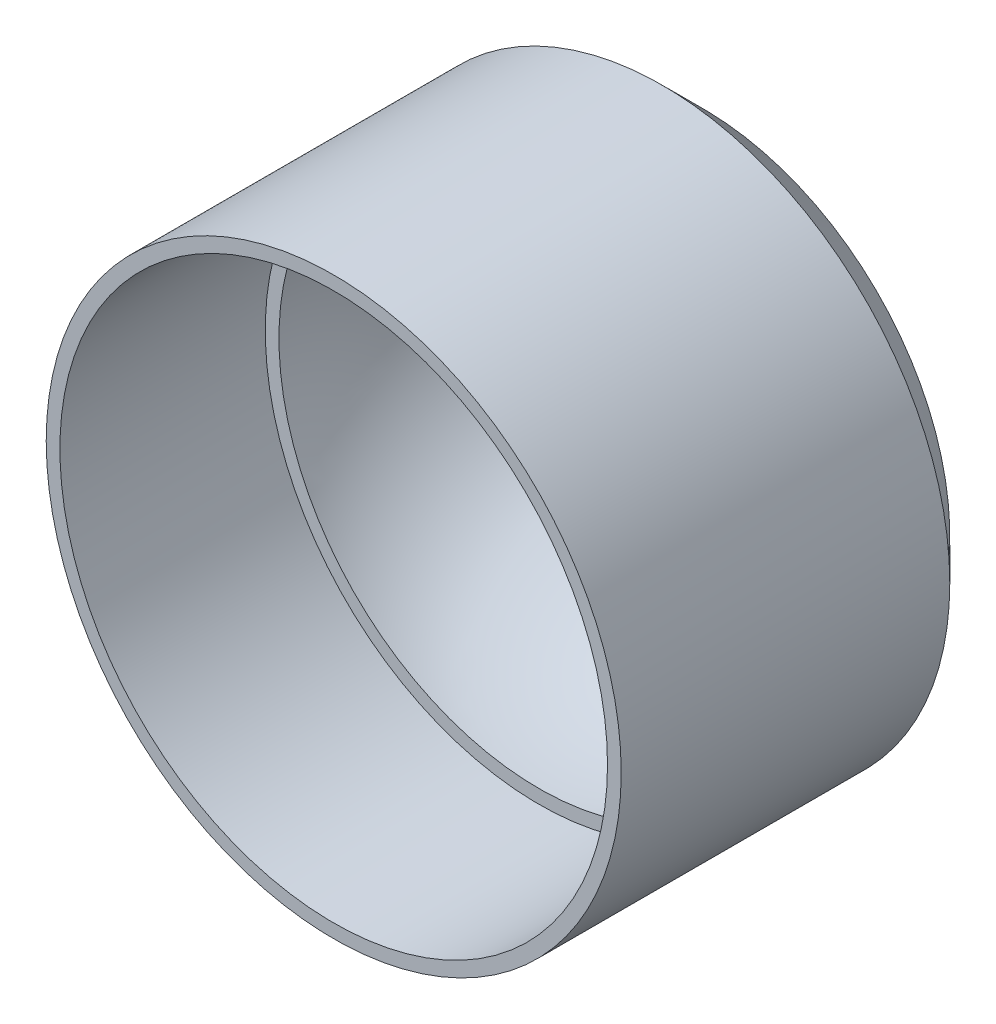
from build123d import *

# Parameters (mm, degrees)
SKETCH1_R           = 21
BOSS_EXTRUDE1_DEPTH = 45
SKETCH8_R           = 19
CUT_EXTRUDE4_DEPTH  = 15
SKETCH2_R           = 20
CUT_EXTRUDE5_DEPTH  = 15
SKETCH6_R           = 5.5
CUT_EXTRUDE6_DEPTH  = 54.916602267
SKETCH10_R          = 21
CUT_EXTRUDE7_DEPTH  = 10
SKETCH13_R          = 21
CUT_EXTRUDE10_DEPTH = 8
CHAMFER4_SIZE       = 3


with BuildPart() as part:
    # Sketch1 → Boss-Extrude1 (new body)
    with BuildSketch(Plane.XY):
        with Locations(Location((0, 0, 0), (0, 0, 180))):
            Circle(SKETCH1_R)
    extrude(amount=BOSS_EXTRUDE1_DEPTH)

    # Sketch8 → Cut-Extrude4 (cut)
    with BuildSketch(Plane.XY.offset(45)):
        Circle(SKETCH8_R)
    extrude(amount=-CUT_EXTRUDE4_DEPTH, mode=Mode.SUBTRACT)

    # Sketch9 → Cut-Revolve2 (revolve, cut)
    with BuildSketch(Plane.XY.offset(30)):
        with BuildLine():
            Line((19, 0), (-19, 0))
            ThreePointArc((-19, 0), (0, 19), (19, 0))
        make_face()
    revolve(axis=Axis((19, 0, 30), (-1, 0, 0)), mode=Mode.SUBTRACT)

    # Sketch2 → Cut-Extrude5 (cut)
    with BuildSketch(Plane.XY.offset(45)):
        Circle(SKETCH2_R)
    extrude(amount=-CUT_EXTRUDE5_DEPTH, mode=Mode.SUBTRACT)

    # Sketch6 → Cut-Extrude6 (cut, through all)
    with BuildSketch(Plane(origin=(0, 0, 0), x_dir=(-1, 0, 0), z_dir=(0, 0, -1))):
        Circle(SKETCH6_R)
    extrude(amount=-CUT_EXTRUDE6_DEPTH, mode=Mode.SUBTRACT)

    # Sketch10 → Cut-Extrude7 (cut)
    with BuildSketch(Plane(origin=(0, 0, 0), x_dir=(-1, 0, 0), z_dir=(0, 0, -1))):
        Circle(SKETCH10_R)
    extrude(amount=-CUT_EXTRUDE7_DEPTH, mode=Mode.SUBTRACT)

    # Sketch13 → Cut-Extrude10 (cut)
    with BuildSketch(Plane(origin=(0, 0, 10), x_dir=(-1, 0, 0), z_dir=(0, 0, -1))):
        Circle(SKETCH13_R)
    extrude(amount=-CUT_EXTRUDE10_DEPTH, mode=Mode.SUBTRACT)

    # Chamfer4
    chamfer4_edges = [part.edges().sort_by_distance(p)[0] for p in [
        (21, 0, 18),
    ]]
    chamfer(chamfer4_edges, length=CHAMFER4_SIZE)


solid = part.part
